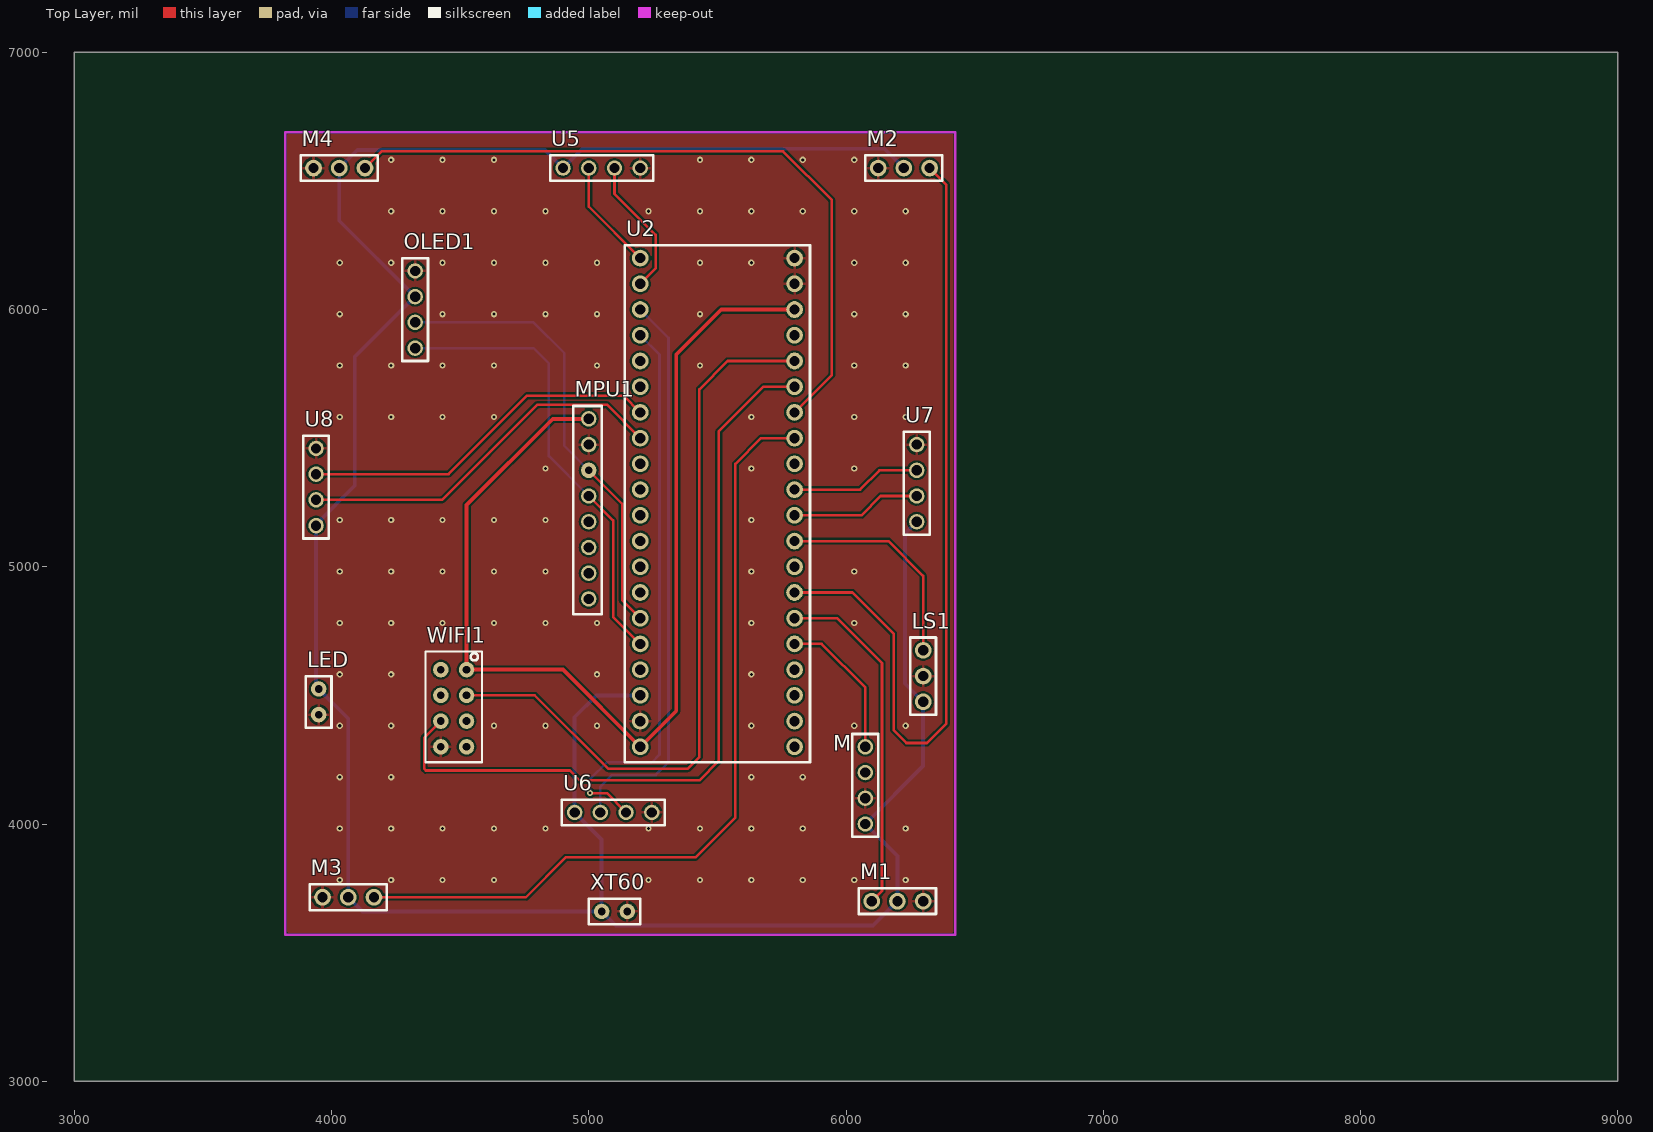
[diagram p0: Top Layer view]
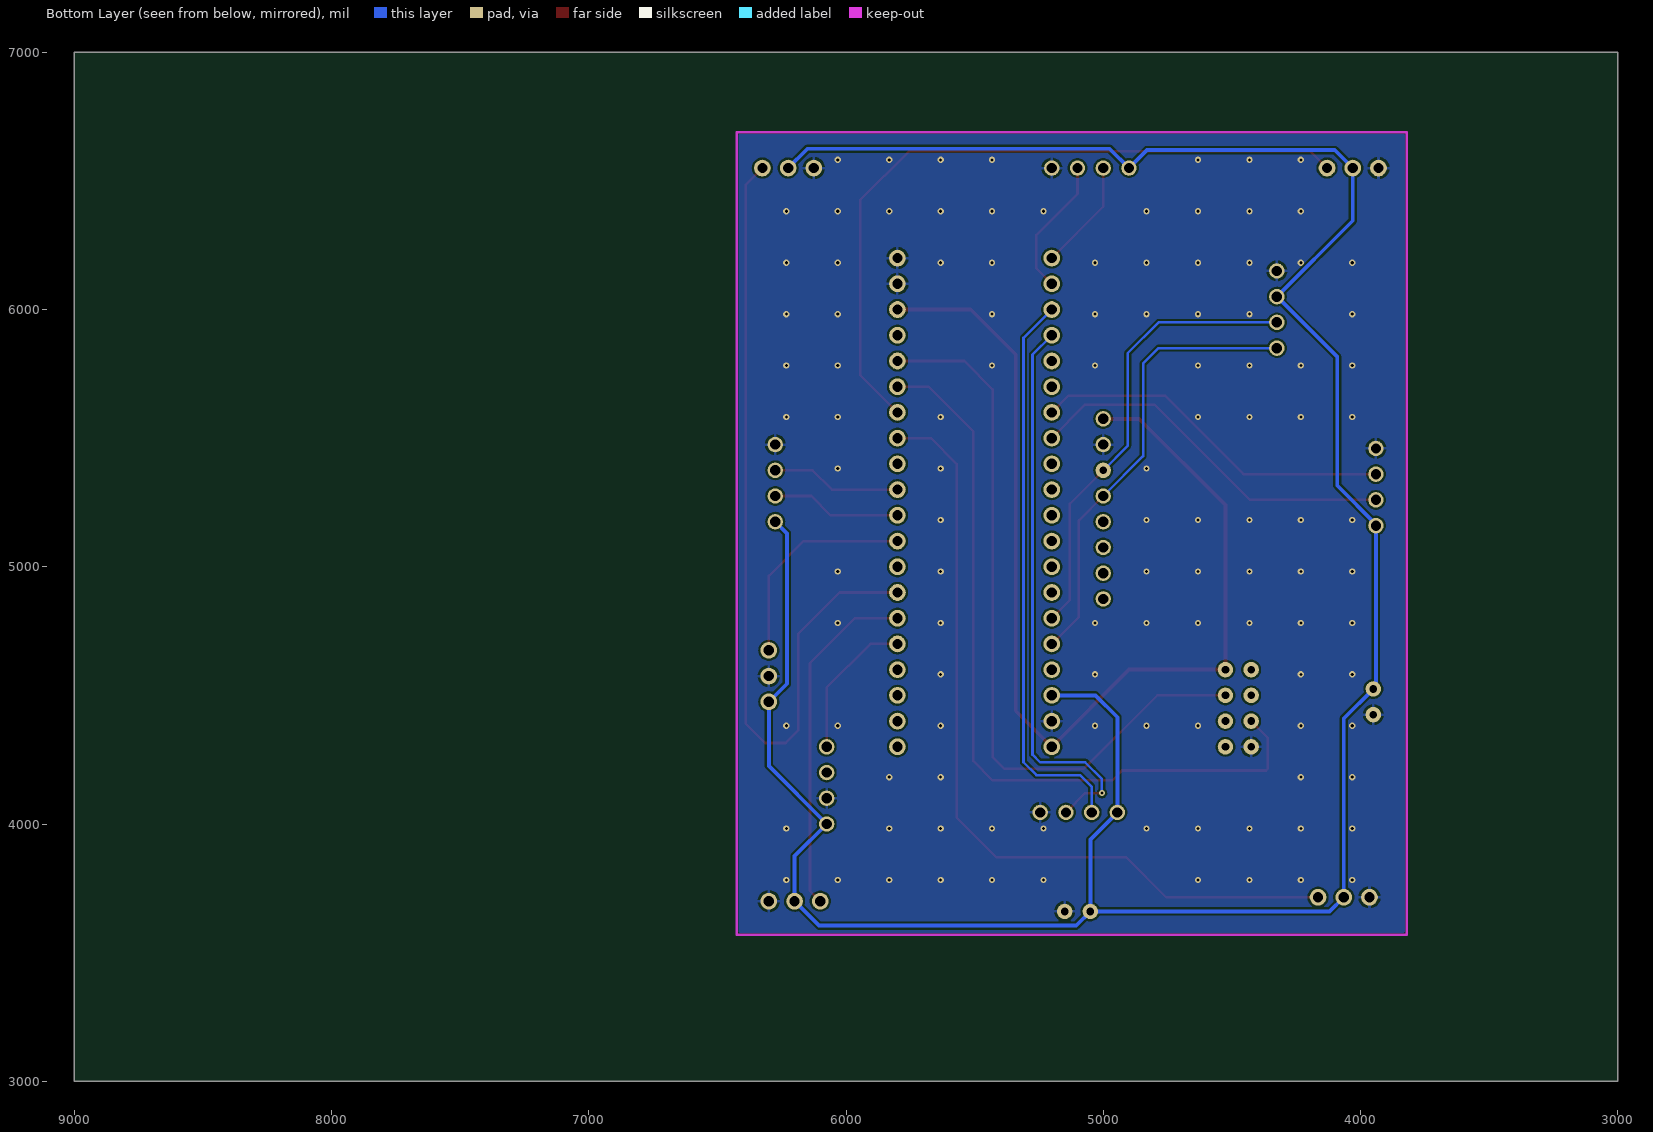
[diagram p1: Bottom Layer view, seen from below]
# Altium PCB MISC51067.pcbdoc
Units mil, origin at the board's own origin, x right, y up, seen from the top; angles counter-clockwise.
Board outline 6000 x 4000 mil, 2 copper layers (Top Layer, Bottom Layer); 16 components, 21 nets, 100 pads, 111 vias.

## Layer stack, top to bottom (the 12.6 mil dielectric is the usual default, probably not edited)
Top Solder Mask Layer: solder mask 0.4, Solder Resist, Dk 3.5
Top Layer: signal copper 1.4
Dielectric 1: surface 12.6, FR-4, Dk 4.8
Bottom Layer: signal copper 1.4
Bottom Solder Mask Layer: solder mask 0.4, Solder Resist, Dk 3.5

## Board outline
3000,7000 3000,3000 9000,3000 9000,7000

## Design rules (kind name [scope] priority, off if disabled: settings)
BoardOutlineClearance Clearance_1 [All] p2: genericclearance=7.87 ignorepadtopadclearanceinfootprint=FALSE except(0: Arc-SplitContinuation Track-SplitContinuation SMDPad-SplitContinuation THPad-SplitContinuation Via-SplitContinuation Fill-SplitContinuation Region-SplitContinuation Poly-SplitContinuation Text-SplitContinuation Hole-SplitContinuation; 6: SMDPad-CutoutEdge THPad-CutoutEdge Via-CutoutEdge Fill-CutoutEdge Region-CutoutEdge Text-CutoutEdge; 6.9: Hole-CutoutEdge; 7.87: Arc-OutlineEdge Track-OutlineEdge SMDPad-OutlineEdge THPad-OutlineEdge Via-OutlineEdge Fill-OutlineEdge Region-OutlineEdge Poly-OutlineEdge Text-OutlineEdge Hole-OutlineEdge Poly-CutoutEdge; 11.8: Arc-CutoutEdge Track-CutoutEdge)
Clearance [All] p1: gap=7.87 ignorepadtopadclearanceinfootprint=FALSE
Creepage creepage [All] p1: checkdistance=0 ignoreinternallayers=TRUE applytopolygonpour=TRUE
DiffPairsRouting [All] p1: maxlimit=10 minlimit=6 mostfreqgap=6 toplayer_minwidth=15 toplayer_prefwidth=15 toplayer_maxwidth=15 toplayer_mingap=10 toplayer_prefgap=10 toplayer_maxgap=10 bottomlayer_minwidth=15 bottomlayer_prefwidth=15 bottomlayer_maxwidth=15 bottomlayer_mingap=10 bottomlayer_prefgap=10 bottomlayer_maxgap=10 maxuncoupledlength=10
HoleToHoleClearance ComponentClearance [All] p1: gap=10 allowstackedmicrovias=TRUE
Length netLength [All] p1: minlimit=0 maxlimit=0
MatchedLengths netLengthTolerance [All] p1: tolerance=1000
PolygonConnect [(InNet('GND'))] p1: connectstyle=Relief reliefconductorwidth=10 reliefentries=4 polygonreliefangle="90 Angle" airgapwidth=10 via.connectstyle=Relief via.reliefconductorwidth=10 via.reliefentries=4 via.polygonreliefangle="90 Angle" via.airgapwidth=10
RoutingVias [All] p1: holewidth=28 width=50 viastyle="Through Hole" minholewidth=1 minwidth=1 maxholewidth=28 maxwidth=50
SolderMaskExpansion [All] p1: expansion=4 istentingtop=FALSE
Width Power_Path [(InNet('3.3V') OR InNet('+5') OR InNet('GND'))] p1: maxlimit=10 minlimit=10 preferedwidth=10 toplayer_minwidth=15 toplayer_maxwidth=25.6 toplayer_prefwidth=25.6 bottomlayer_minwidth=15 bottomlayer_maxwidth=25.6 bottomlayer_prefwidth=25.6
Width [All] p2: maxlimit=10 minlimit=10 preferedwidth=10 toplayer_minwidth=5.9 toplayer_maxwidth=23.6 toplayer_prefwidth=7.9 bottomlayer_minwidth=5.9 bottomlayer_maxwidth=23.6 bottomlayer_prefwidth=7.9
2 further rules are at their usual default settings.

## Components (designator, comment, footprint, x,y, rotation, side; value= is the part's Value field where it differs from the comment)
LED "LED" XT60 3950,4325 r0 top
LS1 "Buzzer" header 6300,4575 r180 top
M "MH-SENSOR" OLED -7525,21800 r180 top
M1 "header_3" header 6200,3700 r90 top
M2 "header_3" header 6225,6550 r270 top
M3 "header_3" header 4065,3715 r90 top
M4 "header_3" header 4030,6550 r90 top
MPU1 "MPU6050" MPU6050 13000,-2225 r0 top
OLED1 "OLED" OLED 17925,-11650 r0 top
U2 "STM32_BluePill" STM32_BluePill_1 5200,6200 r0 top
U5 "HC-SR04" OLED 22700,20150 r90 top
U6 "HC-SR04" OLED 22745,17645 r90 top
U7 "HC-SR04" OLED -7325,22975 r180 top
U8 "HC-SR04" OLED -9660,22960 r180 top
WIFI1 "ESP8266" ESP8266 4425,4500 r270 top
XT60 "XT60" XT60 5250,3660 r90 top

## Footprints (in the part's own frame and the unit in brackets; to place one, negate y for a bottom-side part, rotate by r counter-clockwise, add the part's x,y. Pads: shape width x height; smd on the part's side, far side on the other; paste and mask are expansions set on the pad)
ESP8266 [mil]
  round 60 hole 30: 1(-100,100) 2(0,100) 3(100,100) 4(200,100) 5(-100,0) 6(0,0) 7(100,0) 8(200,0)
  silkscreen extent -170,-60 260,160
header [mil]
  round 65 hole 40: 1(0,100) 2(0,0) 3(0,-100)
  silkscreen extent -50,-150 50,150
MPU6050 [mil]
  round 60 hole 40: 1(-8000,7800) 2(-8000,7700) 5(-8000,7400) 6(-8000,7300) 7(-8000,7200) 8(-8000,7100) ""(-8000,7500)
  round 60 hole 30: 3(-8000,7600)
  silkscreen extent -8060,7040 -7950,7850
OLED [mil]
  round 60 hole 40: 1(-13600,17800) 2(-13600,17700) 3(-13600,17600) 4(-13600,17500)
  silkscreen extent -13650,17450 -13550,17850
STM32_BluePill_1 [mil]
  round 65 hole 40: 1(0,0) 2(0,-100) 3(0,-200) 4(0,-300) 5(0,-400) 6(0,-500) 7(0,-600) 8(0,-700) 9(0,-800) 10(0,-900) 11(0,-1000) 12(0,-1100) 13(0,-1200) 14(0,-1300) 15(0,-1500) 15(0,-1400) 16(0,-1500) 17(0,-1600) 18(0,-1700) 19(0,-1800) 20(0,-1900) 21(600,0) 22(600,-100) 23(600,-200) 24(600,-300) 25(600,-400) 26(600,-500) 27(600,-600) 28(600,-700) 29(600,-800) 30(600,-900) 31(600,-1000) 32(600,-1100) 33(600,-1200) 34(600,-1300) 35(600,-1400) 36(600,-1500) 37(600,-1600) 38(600,-1700) 39(600,-1800) 40(600,-1900)
  silkscreen extent -60,-1960 660,50
XT60 [mil]
  round 60 hole 30: 1(0,200) 2(0,100)
  silkscreen extent -50,50 50,250

## Via types
v1: diameter 24, hole 12, Top Layer to Bottom Layer, 110 vias
v2: diameter 24.02, hole 12, Top Layer to Bottom Layer, 1 vias

## Nets (pads, with @x,y where several pads share a name; then routed paths per layer and width w, separated by ;. In a path a pad name is that pad's centre, name@x,y a point inside that pad or via, vN(x,y) a via of type N, cw(c..) or ccw(c..) an arc to the next point about the centre after c; other vN are vias at no path point)
3.3V: MPU1.1 U2.20 U2.23 WIFI1.1 | length 4168.5
  Top Layer w14.96: MPU1.1 4860,5575 4525,5240 WIFI1.1 4900,4600 U2.20 5340,4440 5340,5825 5515,6000 U2.23
+5: LED.1 LS1.1 M1.2 M2.2 M3.2 M4.2 M.1 OLED1.2 U2.18 U5.1 U6.1 U7.1 U8.1 XT60.1 | length 10459.8
  Bottom Layer w14.96: U2.18 5030,4500 4945,4415 U6.1 5050,3940 XT60.1 ; M2.2 6150,6625 4975,6625 U5.1 4830,6620 4100,6620 M4.2 4030,6345 OLED1.2 4090,5815 4090,5315 3940,5165 U8.1 3940,4535 LED.1 4065,4410 M3.2 4120,3660 XT60.1 ; U7.1 6230,5130 6230,4545 LS1.1 6300,4225 M.1 6200,3875 M1.2 6105,3605 5105,3605 XT60.1
Buzzer_SIG: LS1.3 U2.32 | length 845.9
  Top Layer w10: U2.32 6165,5100 6300,4965 LS1.3
Echo_B: U2.4 U6.3 | length 2196.5
  Top Layer w10: v2(5005,4120) 5070,4120 U6.3
  Bottom Layer w10: v2(5005,4120) 5005,4175 5070,4240 5245,4240 5275,4270 5275,5825 U2.4
Echo_F: U2.2 U5.3 | length 541.1
  Top Layer w10: U5.3 5100,6450 5260,6290 5260,6160 U2.2
Echo_L: U2.7 U8.3 | length 1413.3
  Top Layer w10: U8.3 4455,5360 4760,5665 5135,5665 U2.7
Echo_R: U2.30 U7.3 | length 506.1
  Top Layer w10: U2.30 6055,5300 6130,5375 U7.3
GND: LED.2 LS1.2 M1.3 M2.3 M3.1 M4.1 M.2 MPU1.2 OLED1.1 U2.19 U2.21 U2.22 U5.4 U6.4 U7.4 U8.4 WIFI1.8 XT60.2
  other v1: 4031.97,3781.97 4231.97,3781.97 4431.97,3781.97 4631.97,3781.97 5231.97,3781.97 5431.97,3781.97 5631.97,3781.97 5831.97,3781.97 6031.97,3781.97 6231.97,3781.97 4031.97,3981.97 4231.97,3981.97 4431.97,3981.97 4631.97,3981.97 4831.97,3981.97 5231.97,3981.97 5431.97,3981.97 5631.97,3981.97 5831.97,3981.97 6231.97,3981.97 4031.97,4181.97 4231.97,4181.97 5631.97,4181.97 5831.97,4181.97 4031.97,4381.97 4231.97,4381.97 4631.97,4381.97 4831.97,4381.97 5031.97,4381.97 5631.97,4381.97 6031.97,4381.97 6231.97,4381.97 4031.97,4581.97 4231.97,4581.97 5031.97,4581.97 5631.97,4581.97 4031.97,4781.97 4231.97,4781.97 4431.97,4781.97 4631.97,4781.97 4831.97,4781.97 5031.97,4781.97 5631.97,4781.97 6031.97,4781.97 4031.97,4981.97 4231.97,4981.97 4431.97,4981.97 4631.97,4981.97 4831.97,4981.97 5631.97,4981.97 6031.97,4981.97 4031.97,5181.97 4231.97,5181.97 4431.97,5181.97 4631.97,5181.97 4831.97,5181.97 5631.97,5181.97 4831.97,5381.97 5631.97,5381.97 6031.97,5381.97 4031.97,5581.97 4231.97,5581.97 4431.97,5581.97 4631.97,5581.97 5631.97,5581.97 6031.97,5581.97 6231.97,5581.97 4031.97,5781.97 4231.97,5781.97 4431.97,5781.97 4631.97,5781.97 5031.97,5781.97 5431.97,5781.97 6031.97,5781.97 6231.97,5781.97 4031.97,5981.97 4431.97,5981.97 4631.97,5981.97 4831.97,5981.97 5031.97,5981.97 5431.97,5981.97 6031.97,5981.97 6231.97,5981.97 4031.97,6181.97 4231.97,6181.97 4431.97,6181.97 4631.97,6181.97 4831.97,6181.97 5031.97,6181.97 5431.97,6181.97 5631.97,6181.97 6031.97,6181.97 6231.97,6181.97 4231.97,6381.97 4431.97,6381.97 4631.97,6381.97 4831.97,6381.97 5231.97,6381.97 5431.97,6381.97 5631.97,6381.97 5831.97,6381.97 6031.97,6381.97 6231.97,6381.97 4231.97,6581.97 4431.97,6581.97 4631.97,6581.97 5431.97,6581.97 5631.97,6581.97 5831.97,6581.97 6031.97,6581.97
I2C_SCL: MPU1.3 OLED1.3 U2.15@5200,4800 | length 1781.9
  Top Layer w10: MPU1.3 5130,5245 5130,4870 U2.15@5200,4800
  Bottom Layer w10: OLED1.3 4785,5950 4905,5830 4905,5470 MPU1.3
I2C_SDA: MPU1. OLED1.4 U2.15@5200,4700 U2.16 | length 1781.9
  Top Layer w10: MPU1. 5095,5180 5095,4805 U2.16
  Bottom Layer w10: OLED1.4 4785,5850 4845,5790 4845,5430 MPU1.
M1_SIG: M1.1 U2.35 | length 1354.1
  Top Layer w10: U2.35 5965,4800 6140,4625 6140,3740 M1.1
M2_SIG: M2.1 U2.34 | length 3270
  Top Layer w10: U2.34 6025,4900 6185,4740 6185,4365 6235,4315 6315,4315 6390,4390 6390,6485 M2.1
M3_SIG: M3.3 U2.28 | length 3179.8
  Top Layer w10: M3.3 4755,3715 4910,3870 5415,3870 5570,4025 5570,5400 5670,5500 U2.28
M4_SIG: M4.3 U2.27 | length 2805.7
  Top Layer w10: M4.3 4195,6615 5755,6615 5945,6425 5945,5745 U2.27
PA0: M.4 U2.36 | length 575.4
  Top Layer w10: U2.36 5905,4700 6075,4530 M.4
Trig_B: U2.3 U6.2 | length 2209.9
  Bottom Layer w10: U6.2 5045,4145 5090,4190 5260,4190 5310,4240 5310,5890 U2.3
Trig_F: U2.1 U5.2 | length 432.8
  Top Layer w10: U5.2 5000,6400 U2.1
Trig_L: U2.8 U8.2 | length 1467.1
  Top Layer w10: U8.2 4430,5260 4800,5630 5070,5630 U2.8
Trig_R: U2.31 U7.2 | length 506.1
  Top Layer w10: U2.31 6060,5200 6135,5275 U7.2
USART2_RX: U2.25 WIFI1.2 | length 2887.3
  Top Layer w10: WIFI1.2 4790,4500 5075,4215 5385,4215 5430,4260 5430,5690 5540,5800 U2.25
USART2_TX: U2.26 WIFI1.7 | length 3054.1
  Top Layer w10: WIFI1.7 4360,4335 4360,4215 4367.07,4207.93 4927.07,4207.93 4965,4170 5430,4170 5505,4245 5505,5525 5680,5700 U2.26
pads on no net: M.3 MPU1.5 MPU1.6 MPU1.7 MPU1.8 U2.5 U2.6 U2.9 U2.10 U2.11 U2.12 U2.13 U2.14 U2.17 U2.24 U2.29 U2.33 U2.37 U2.38 U2.39 U2.40 WIFI1.3 WIFI1.4 WIFI1.5 WIFI1.6

## Polygon pours and split planes (outlines as drawn)
GND on Top Layer (solid, remove dead copper, pour order 0): 3315,6915 3315,3310 6950,3310 6950,6915
GND on Bottom Layer (solid, remove dead copper, pour order 2): 3655,6820 3655,3255 6740,3255 6740,6820

## Keep-outs
Board Outline Layer:
  lines w10: 3820,3570 3820,6689.61 6425,6689.61 6425,3570 3820,3570